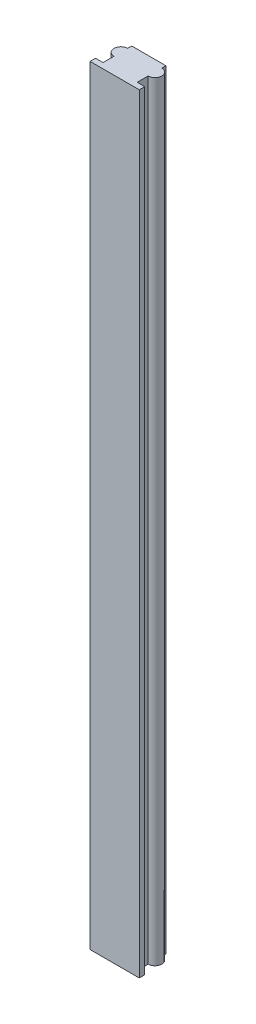
from build123d import *

# Parameters (mm, degrees)
EXTRUDE_1_DEPTH = 563


with BuildPart() as part:
    # 草图1 → 凸台-拉伸1 (new body)
    with BuildSketch(Plane(origin=(0, 0, 0), x_dir=(1, 0, 0), z_dir=(0, 1, 0))):
        with BuildLine():
            Line((-12.5, 5), (-12.5, 8))
            Line((-12.5, 8), (12.5, 8))
            Line((12.5, 8), (12.5, 5))
            ThreePointArc((12.5, 5), (17.5, 0), (12.5, -5))
            Line((12.5, -5), (12.5, -13))
            Line((12.5, -13), (18, -13))
            Line((18, -13), (18, -17))
            Line((18, -17), (-18, -17))
            Line((-18, -17), (-18, -13))
            Line((-18, -13), (-12.5, -13))
            Line((-12.5, -13), (-12.5, -5))
            ThreePointArc((-12.5, -5), (-17.5, 0), (-12.5, 5))
        make_face()
    extrude(amount=EXTRUDE_1_DEPTH)


solid = part.part
